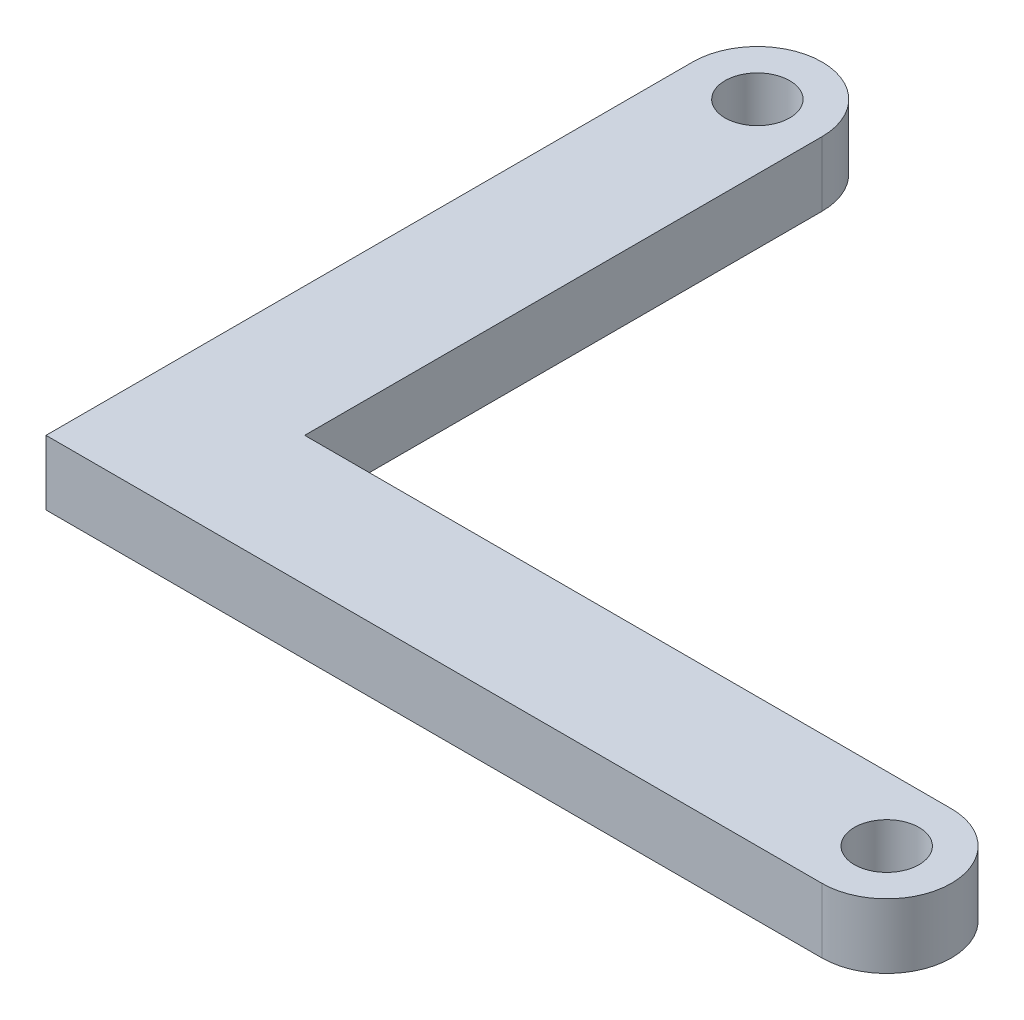
from build123d import *

# Parameters (mm, degrees)
SKETCH1_R           = 2.5
BOSS_EXTRUDE1_DEPTH = 5


with BuildPart() as part:
    # Sketch1 → Boss-Extrude1 (new body)
    with BuildSketch(Plane(origin=(0, 0, 0), x_dir=(1, 0, 0), z_dir=(0, 1, 0))):
        with BuildLine():
            Line((-25, -5), (25, -5))
            ThreePointArc((25, -5), (30, 0), (25, 5))
            Line((25, 5), (-25, 5))
            Line((-25, 5), (-25, 45))
            ThreePointArc((-25, 45), (-30, 50), (-35, 45))
            Line((-35, 45), (-35, -5))
            Line((-35, -5), (-25, -5))
        make_face()
        with Locations(Location((25, 0, 0), (0, 0, 270))):
            Circle(SKETCH1_R, mode=Mode.SUBTRACT)
        with Locations(Location((-30, 45, 0), (0, 0, 270))):
            Circle(SKETCH1_R, mode=Mode.SUBTRACT)
    extrude(amount=BOSS_EXTRUDE1_DEPTH)


solid = part.part
